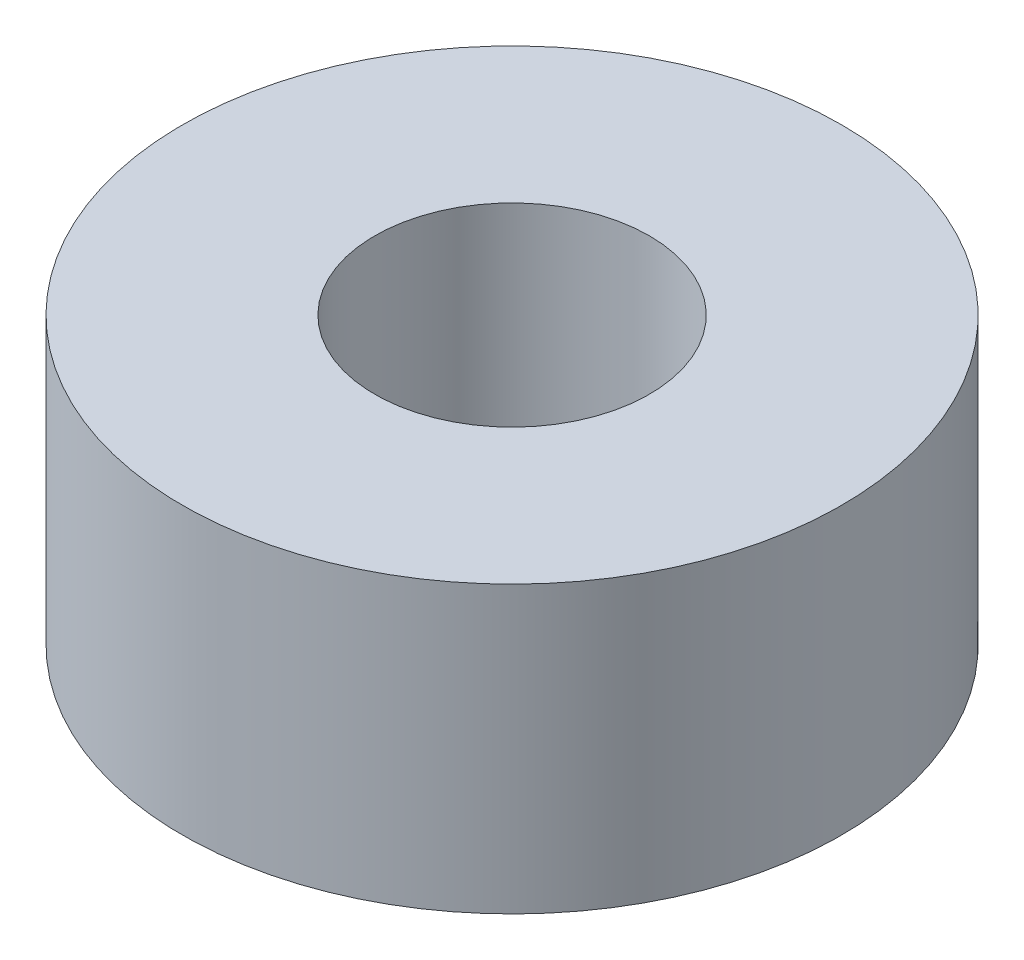
from build123d import *


with BuildPart() as part:
    # Sketch1 → Revolve1 (revolve)
    with BuildSketch(Plane.XY, mode=Mode.PRIVATE) as revolve1_sk:
        Polygon((25, 0), (25, 60), (60, 60), (60, 8), (35, 8), (35, 0), align=None)
    revolve(revolve1_sk.sketch.rotate(Axis((0, 0, 0), (0, 1, 0)), 90), axis=Axis((0, 0, 0), (0, 1, 0)))


solid = part.part
